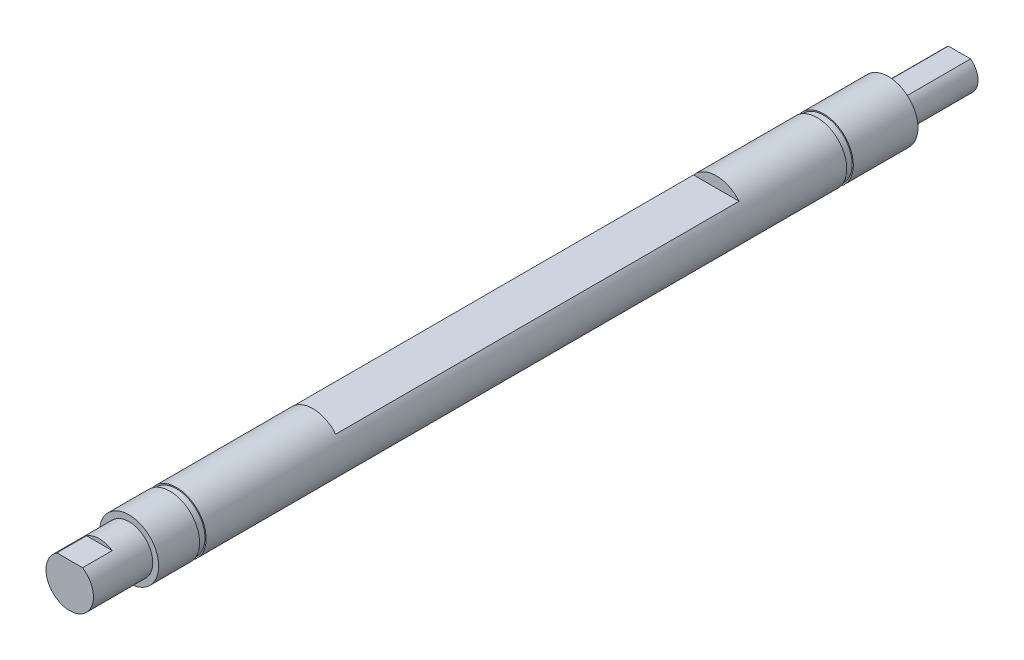
SolidWorks part; units mm, degrees
ref_plane "Front Plane" through (0, 0, 0) normal (0, 0, 1) x (1, 0, 0)
ref_plane "Top Plane" through (0, 0, 0) normal (0, 1, 0) x (1, 0, 0)
ref_plane "Right Plane" through (0, 0, 0) normal (1, 0, 0) x (0, 0, -1)
sketch "Sketch1" plane through (0, 0, 0) normal (0, 0, 1) x (1, 0, 0)
  circle A0 centre (0, 0) radius 5
  dimension "D1" = 10
extrude "Boss-Extrude1" add sketch "Sketch1" along normal mid plane 150
sketch "Sketch2" plane through (0, 0, 0) normal (1, 0, 0) x (0, 0, -1)
  line L0 (-75, -5) -> (75, -5) construction
  line L1 (-34, 17.7355) -> (34, 17.7355)
  line L2 (-34, 17.7355) -> (-34, 3.2)
  line L3 (-34, 3.2) -> (34, 3.2)
  line L4 (34, 17.7355) -> (34, 3.2)
  line L5 (0, 0) -> (0, 26.4378) construction
  dimension "D1" = 8.2
  dimension "D2" = 68
extrude "Cut-Extrude1" cut sketch "Sketch2" against normal through all both and the other way through all
sketch "Sketch3" plane through (0, 0, -75) normal (0, 0, -1) x (-1, 0, 0)
  circle A0 centre (0, 0) radius 3.125
  circle A1 centre (0, 0) radius 5 construction
  circle A2 centre (0, 0) radius 5
  dimension "D1" = 6.25
extrude "Cut-Extrude2" cut sketch "Sketch3" against normal blind 12
sketch "Sketch4" plane through (0, 0, -75) normal (0, 0, -1) x (-1, 0, 0)
  line L0 (-1.9572, 2.5) -> (1.9572, 2.5)
  arc A0 (-1.9572, 2.5) -> (1.9572, 2.5) centre (0, 0) ccw
  dimension "D1" = 6.35
  dimension "D2" = 2.5
extrude "Cut-Extrude3" cut sketch "Sketch4" against normal blind 12 flip side to cut
sketch "Sketch5" plane through (0, 0, 75) normal (0, 0, 1) x (1, 0, 0)
  circle A0 centre (0, 0) radius 5 construction
  circle A1 centre (0, 0) radius 5 construction
  circle A2 centre (0, 0) radius 4
  dimension "D1" = 8
extrude "Cut-Extrude4" cut sketch "Sketch5" against normal blind 10 flip side to cut
sketch "Sketch6" plane through (0, 0, 75) normal (0, 0, 1) x (1, 0, 0)
  line L1 (-5.0162, 4.6048) -> (5.5479, 4.6048)
  line L2 (-5.0162, 4.6048) -> (-5.0162, 3.3608)
  line L3 (-5.0162, 3.3608) -> (5.5479, 3.3608)
  line L4 (5.5479, 4.6048) -> (5.5479, 3.3608)
extrude "Cut-Extrude5" cut sketch "Sketch6" against normal blind 5
sketch "Sketch21" plane through (0, 1.7837, -63) normal (0, 0, -1) x (-1, 0, 0)
  line L0 (0, -1.7837) -> (5, -1.7837) construction
  circle A0 centre (0, -1.7837) radius 5
  circle A2 centre (0, -1.7837) radius 5 construction
  point P2 (5, -1.7837)
  dimension "D1" = 10
ref_plane "Plane1" through (-5, 0, -63) normal (0, 1, 0) x (1, 0, 0)
sketch "Sketch31" plane through (-100, 0, -63) normal (0, 1, 0) x (0, 0, 1)
  line L0 (0, 100) -> (33.5023, 100) construction
  line L2 (10.9, 95) -> (12, 95)
  line L3 (10.9, 95) -> (10.9, 95.2)
  line L4 (10.9, 95.2) -> (12, 95.2)
  line L5 (12, 95) -> (12, 95.2)
  line L6 (0, 105) -> (0, 95) construction
  dimension "D1" = 1.1
  dimension "D2" = 4.8
  dimension "D3" = 12
revolve "Cut-Revolve1" cut sketch "Sketch31" angle 360 about L0
other "Shaft Retaining Ring Library <1>"
sketch "Sketch22" plane through (-4, 0, 65) normal (0, 0, 1) x (1, 0, 0)
  line L0 (4, 0) -> (9, 0) construction
  circle A0 centre (4, 0) radius 5
  circle A2 centre (4, 0) radius 5 construction
  point P2 (9, 0)
  dimension "D1" = 10
ref_plane "Plane11" through (5, 0, 65) normal (0, 1, 0) x (1, 0, 0)
sketch "Sketch32" plane through (100, 0, 65) normal (0, 1, 0) x (0, 0, -1)
  line L0 (0, 100) -> (33.5023, 100) construction
  line L2 (6.9, 95) -> (8, 95)
  line L3 (6.9, 95) -> (6.9, 95.2)
  line L4 (6.9, 95.2) -> (8, 95.2)
  line L5 (8, 95) -> (8, 95.2)
  line L6 (0, 105) -> (0, 95) construction
  dimension "D1" = 1.1
  dimension "D2" = 4.8
  dimension "D3" = 8
revolve "Cut-Revolve11" cut sketch "Sketch32" angle 360 about L0
other "Shaft Retaining Ring Library <2>"
